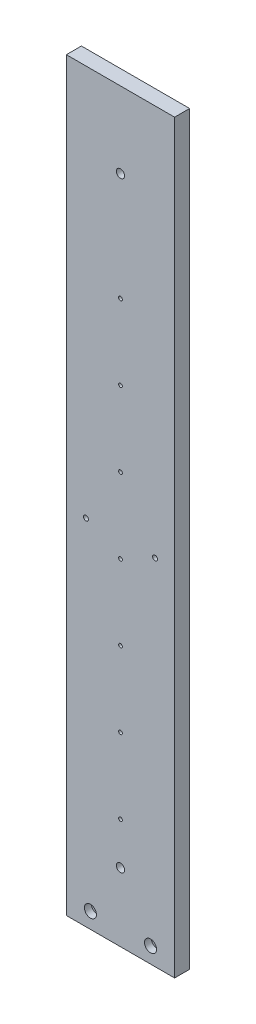
SolidWorks part; units mm, degrees
ref_plane "前视基准面" through (0, 0, 0) normal (0, 0, 1) x (1, 0, 0)
ref_plane "上视基准面" through (0, 0, 0) normal (0, 1, 0) x (1, 0, 0)
ref_plane "右视基准面" through (0, 0, 0) normal (1, 0, 0) x (0, 0, -1)
sketch "草图1" plane through (0, 0, 0) normal (0, 0, 1) x (1, 0, 0)
  line L1 (-36, 248) -> (36, 248)
  line L2 (-36, 248) -> (-36, -248)
  line L3 (-36, -248) -> (36, -248)
  line L4 (36, 248) -> (36, -248)
  line L5 (-36, 248) -> (36, -248) construction
  line L6 (-36, -248) -> (36, 248) construction
  point P0 (0, 0)
  dimension "D1" = 496
  dimension "D2" = 72
extrude "凸台-拉伸1" add sketch "草图1" along normal blind 10
hole_wizard "打孔尺寸根据内六角圆柱头螺钉的类型2" positions "草图6" profile "草图5" counterbore size "M5" standard "Gb" end condition through all
sketch "草图6" plane through (0, 0, 0) normal (0, 0, -1) x (-1, 0, 0)
  point P0 (0, -202.5)
  point P3 (0, 197.5)
sketch "草图5" plane through (0, -202.5, 0) normal (1, 0, 0) x (0, 1, 0)
  line L0 (0, 0) -> (0, 10)
  line L1 (0, 10) -> (2.75, 10)
  line L3 (2.75, 10) -> (2.75, 5.7)
  line L4 (2.75, 5.7) -> (5, 5.7)
  line L5 (5, 5.7) -> (5, 0)
  line L7 (5, 0) -> (0, 0)
  line L11 (0, -6.35) -> (0, 107.95) construction
  dimension "通孔孔直径" = 5.5
  dimension "通孔孔深度" = 10
  dimension "柱形沉头孔直径" = 10
  dimension "柱形沉头孔深度" = 5.7
hole_wizard "打孔尺寸根据内六角圆柱头螺钉的类型4" positions "草图16" profile "草图15" counterbore size "M5" standard "Gb"
sketch "草图16" plane through (0, 0, 0) normal (0, 0, -1) x (-1, 0, 0)
  line L0 (-36, -248) -> (-36, 248) construction
  line L1 (-36, 248) -> (36, 248) construction
  point P0 (4, -14.5)
  dimension "D1" = 40
  dimension "D2" = 262.5
sketch "草图15" plane through (-4, -14.5, 0) normal (1, 0, 0) x (0, 1, 0)
  line L0 (0, 0) -> (0, 10)
  line L1 (0, 10) -> (2.75, 10)
  line L3 (2.75, 10) -> (2.75, 5.7)
  line L4 (2.75, 5.7) -> (5, 5.7)
  line L5 (5, 5.7) -> (5, 0)
  line L7 (5, 0) -> (0, 0)
  line L11 (0, -6.35) -> (0, 107.95) construction
  dimension "通孔孔直径" = 5.5
  dimension "通孔孔深度" = 10
  dimension "柱形沉头孔直径" = 10
  dimension "柱形沉头孔深度" = 5.7
hole_wizard "打孔尺寸根据内六角圆柱头螺钉的类型0" positions "草图20" profile "草图19" counterbore size "M4" standard "Gb" end condition through all
sketch "草图20" plane through (0, 0, 10) normal (0, 0, 1) x (1, 0, 0)
  line L0 (-36, -248) -> (36, -248) construction
  line L1 (36, -248) -> (36, 248) construction
  point P0 (-20, -237.5)
  point P3 (20, -237.5)
  dimension "D1" = 40
  dimension "D2" = 10.5
  dimension "D3" = 16
sketch "草图19" plane through (-20, -237.5, 10) normal (1, 0, 0) x (0, -1, 0)
  line L0 (0, 0) -> (0, 10)
  line L1 (0, 10) -> (2.25, 10)
  line L3 (2.25, 10) -> (2.25, 4.6)
  line L4 (2.25, 4.6) -> (4, 4.6)
  line L5 (4, 4.6) -> (4, 0)
  line L7 (4, 0) -> (0, 0)
  line L11 (0, -6.35) -> (0, 107.95) construction
  dimension "通孔孔直径" = 4.5
  dimension "通孔孔深度" = 10
  dimension "柱形沉头孔直径" = 8
  dimension "柱形沉头孔深度" = 4.6
hole_wizard "M4 螺纹孔2" positions "草图22" profile "草图21" tap size "M4" standard "Iso"
sketch "草图22" plane through (0, -248, 0) normal (0, -1, 0) x (-1, 0, 0)
  line L0 (36, 0) -> (-36, 0) construction
  line L1 (-36, -10) -> (-36, 0) construction
  point P0 (-12, -5)
  point P2 (-29, -5)
  dimension "D1" = 5
  dimension "D2" = 7
  dimension "D3" = 17
sketch "草图21" plane through (12, -248, 5) normal (1, 0, 0) x (0, 0, -1)
  line L0 (0, 0) -> (0, 10.9914)
  line L1 (0, 10.9914) -> (1.65, 10)
  line L2 (1.65, 10) -> (1.65, 0)
  line L5 (1.65, 0) -> (0, 0)
  line L10 (0, 10.9914) -> (-1.65, 10) construction
  line L11 (0, -6.35) -> (0, 107.95) construction
  dimension "螺纹孔钻头直径" = 3.3
  dimension "螺纹孔钻头深度" = 10
  dimension "导头角度" = 118
cosmetic thread "孔螺蚊线8" parameters "D1"=8, "D2"=4
cosmetic thread "孔螺蚊线9" parameters "D1"=8, "D2"=4
hole_wizard "M4 螺纹孔3" positions "草图24" profile "草图23" tap size "M4" standard "Iso" end condition through all
sketch "草图24" plane through (0, 0, 0) normal (0, 0, -1) x (-1, 0, 0)
  line L0 (-23, -12.5) -> (23, -12.5) construction
  line L2 (0, -1.5458) -> (0, -23.4542) construction
  point P0 (-23, -12.5)
  point P2 (23, -12.5)
  point P13 (0, -12.5)
  dimension "D1" = 46
sketch "草图23" plane through (23, -12.5, 0) normal (1, 0, 0) x (0, 1, 0)
  line L0 (0, 0) -> (0, 10)
  line L1 (0, 10) -> (1.65, 10)
  line L2 (1.65, 10) -> (1.65, 0)
  line L5 (1.65, 0) -> (0, 0)
  line L11 (0, -6.35) -> (0, 107.95) construction
  dimension "通孔螺纹孔钻头直径" = 3.3
  dimension "通孔螺纹孔钻头深度" = 10
cosmetic thread "孔螺蚊线10" parameters "D2"=4
cosmetic thread "孔螺蚊线11" parameters "D2"=4
hole_wizard "M3 螺纹孔1" positions "草图26" profile "草图25" tap size "M3" standard "Iso" end condition through all
sketch "草图26" plane through (0, 0, 0) normal (0, 0, -1) x (-1, 0, 0)
  point P0 (0, -174.5)
  point P3 (0, -124.5)
  point P6 (0, -74.5)
  point P9 (0, -24.5)
  point P12 (0, 25.5)
  point P15 (0, 75.5)
  point P18 (0, 125.5)
sketch "草图25" plane through (0, -174.5, 0) normal (1, 0, 0) x (0, 1, 0)
  line L0 (0, 0) -> (0, 10)
  line L1 (0, 10) -> (1.25, 10)
  line L2 (1.25, 10) -> (1.25, 0)
  line L5 (1.25, 0) -> (0, 0)
  line L11 (0, -6.35) -> (0, 107.95) construction
  dimension "螺纹线主直径" = 2.5
  dimension "通孔螺纹孔钻头深度" = 10
